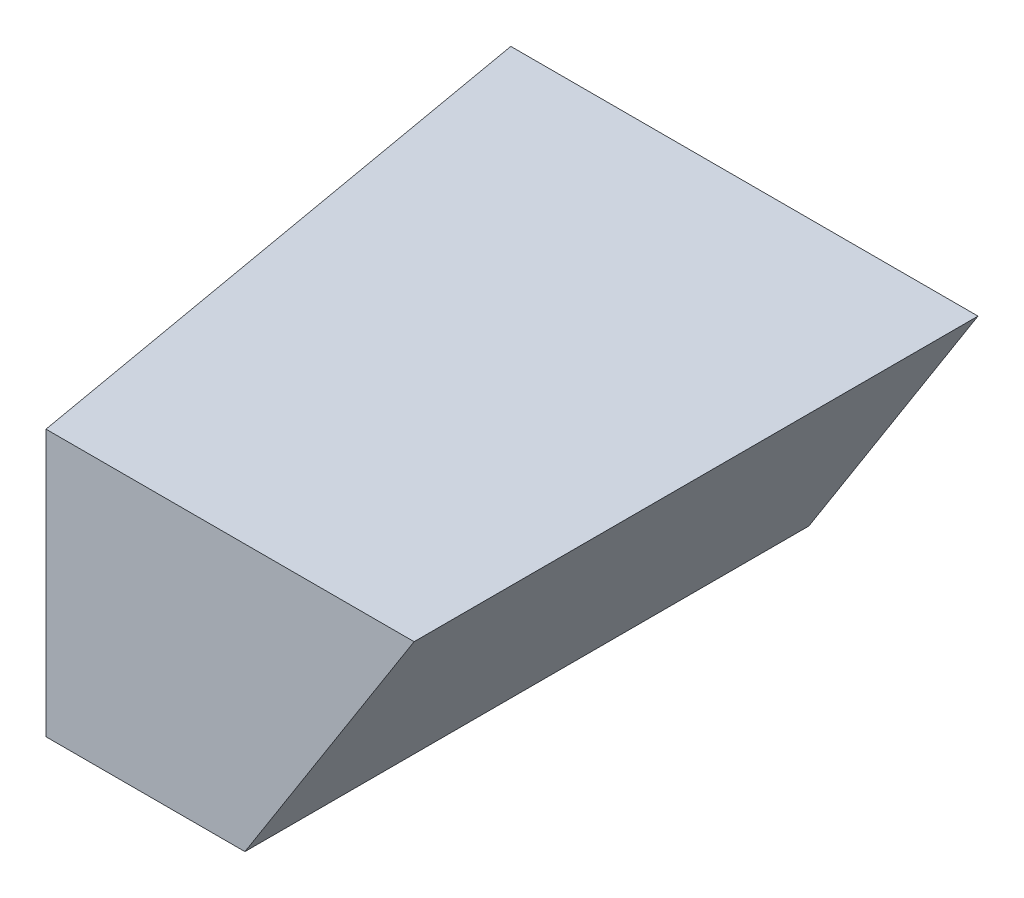
from build123d import *

# Parameters (mm, degrees)
EXTRUDE_1_DEPTH     = 3.175
CUT_EXTRUDE_1_DEPTH = 3.175


with BuildPart() as part:
    # 草图1 → 凸台-拉伸1 (new body)
    with BuildSketch(Plane.XY):
        Polygon((-4.407915319, 5), (-7.407915319, 5), (-7.407915319, 6.5), (-3.455415319, 6.5), align=None)
    extrude(amount=EXTRUDE_1_DEPTH)

    # 草图3 → 切除-拉伸1 (cut)
    with BuildSketch(Plane.XZ.offset(-5)):
        Polygon((-7.407915319, 0), (-6.085915319, 0), (-5.527915319, 3.175), (-7.407915319, 3.175), align=None)
    extrude(amount=-CUT_EXTRUDE_1_DEPTH, mode=Mode.SUBTRACT)


solid = part.part
